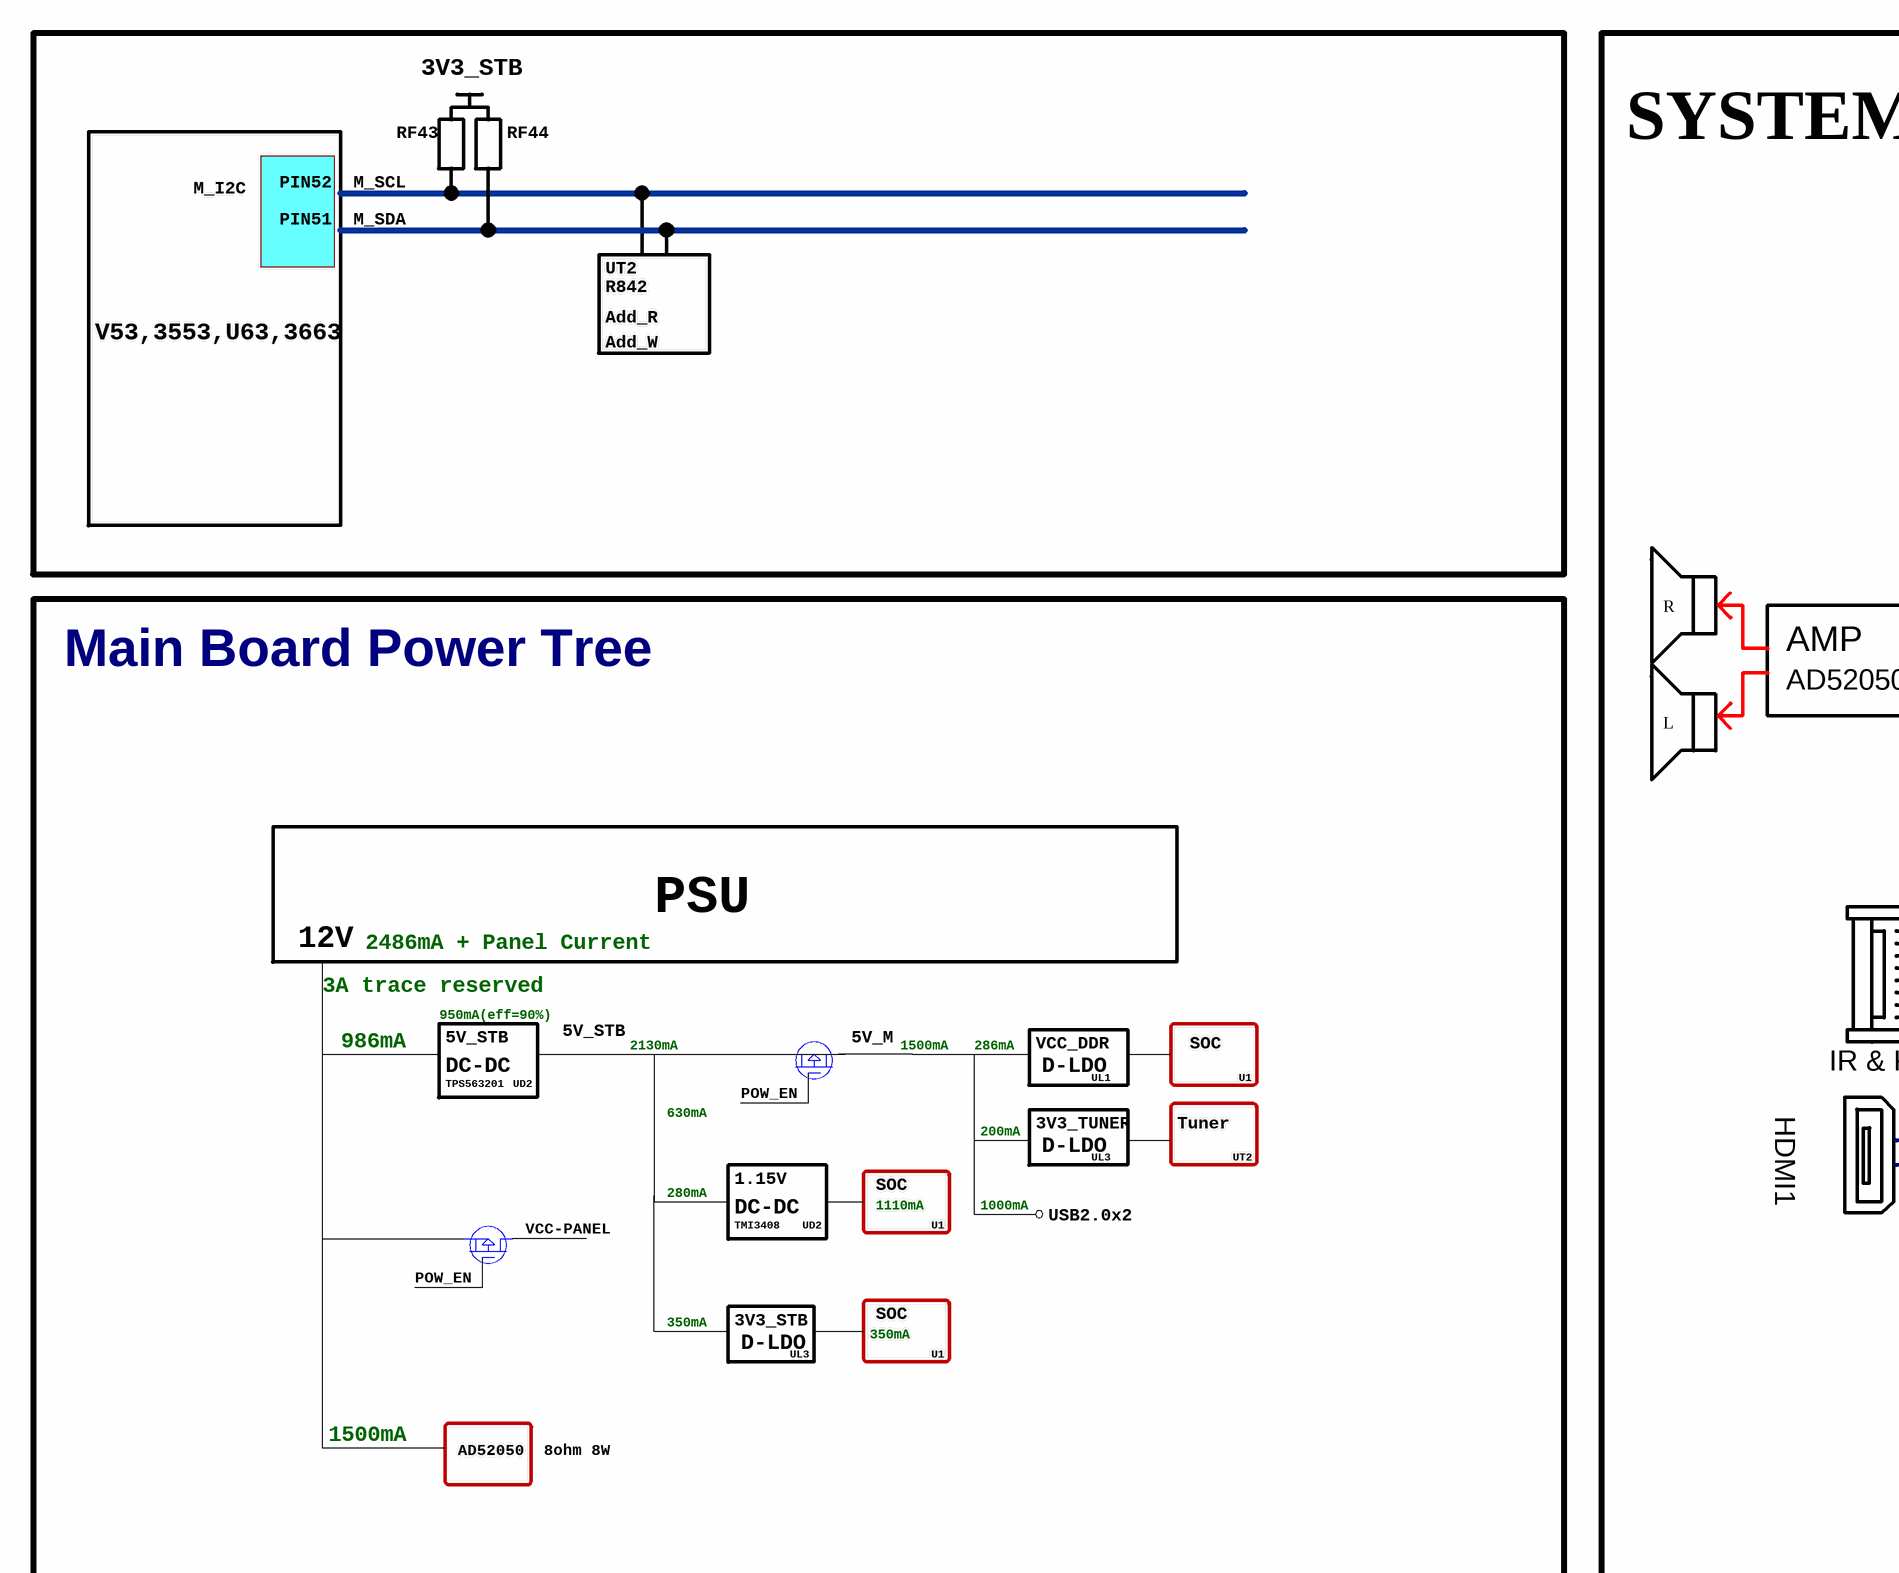
[diagram p0: MISC116569-14.SchDoc, left]
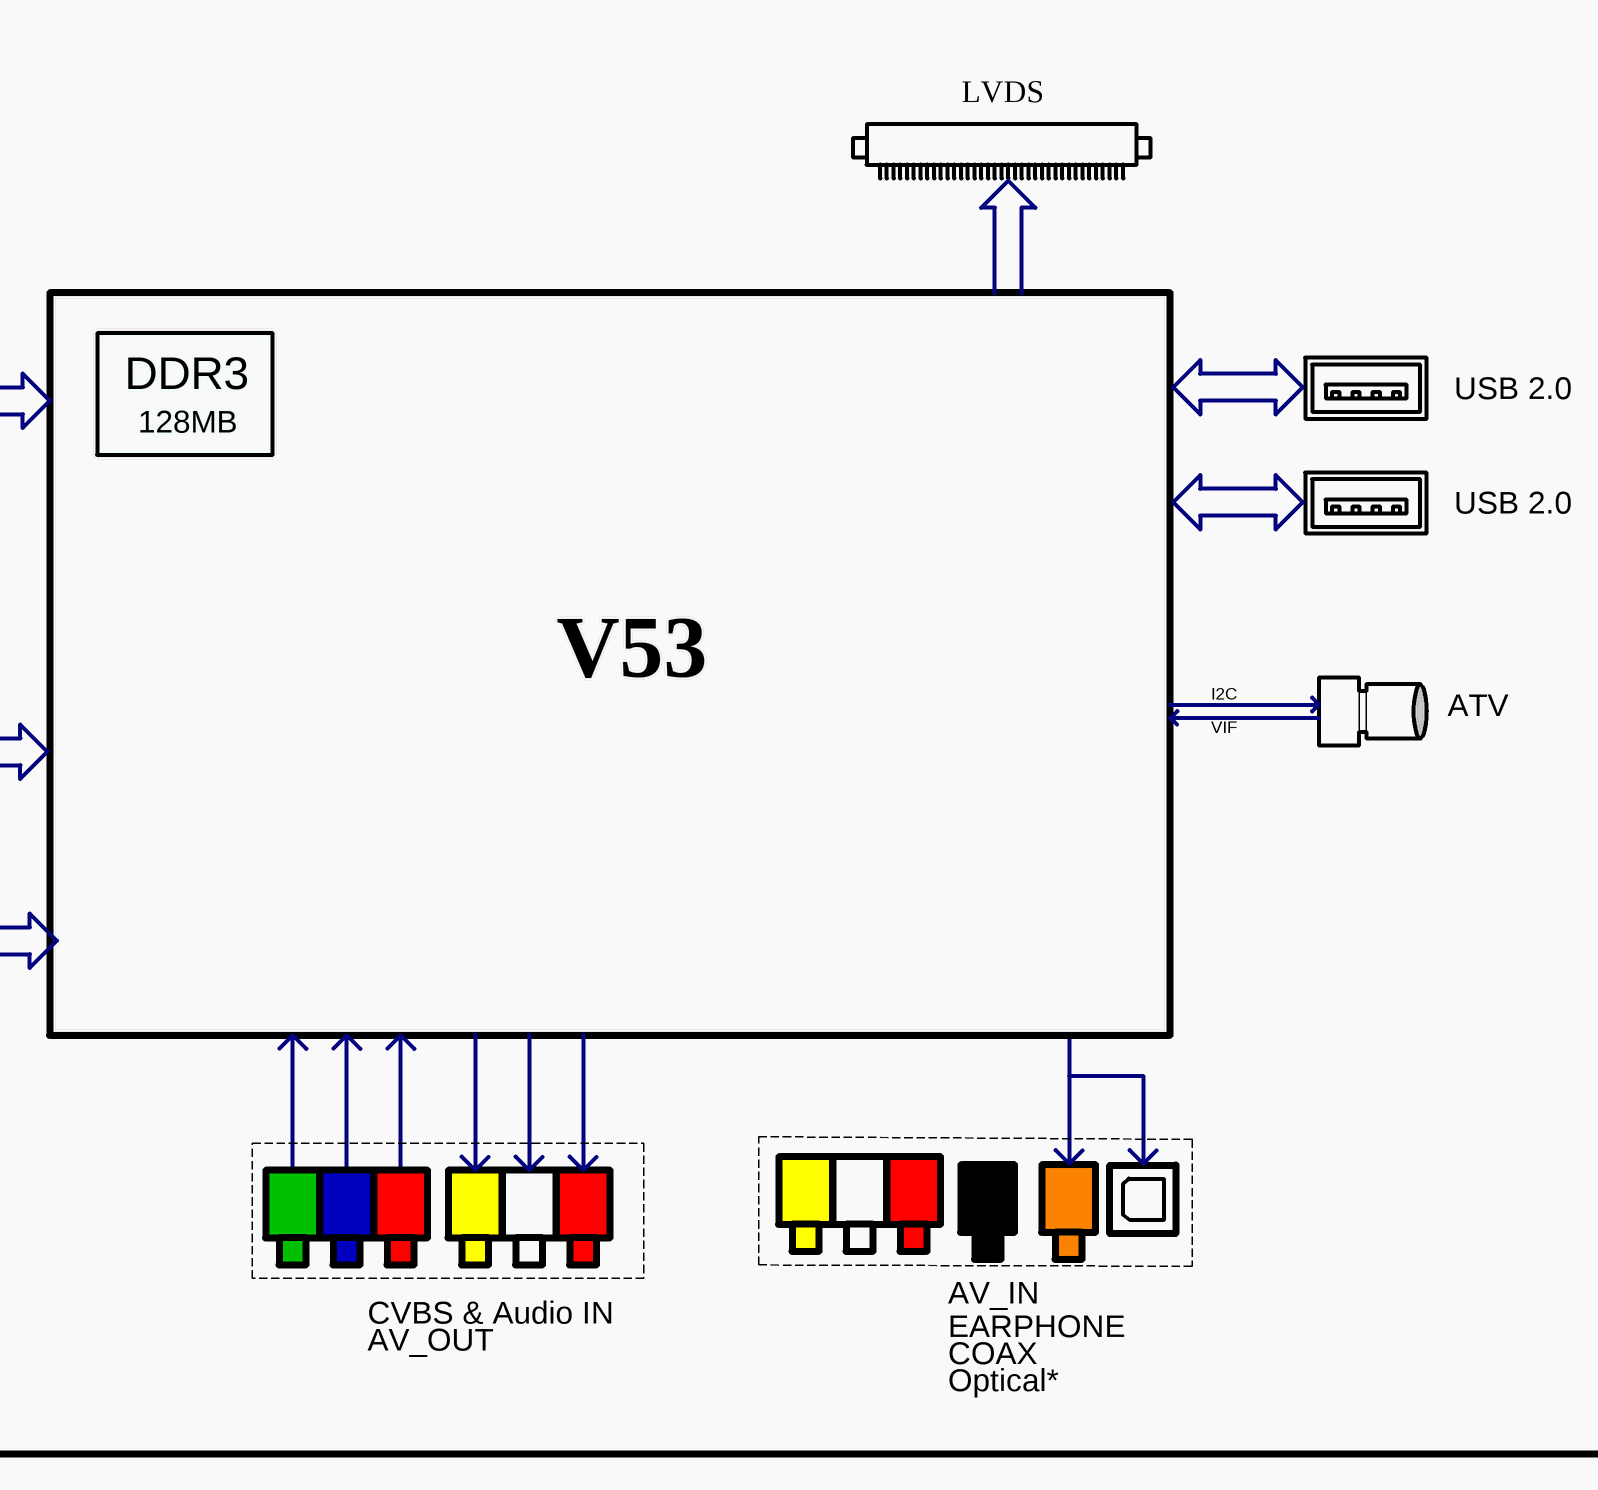
[diagram p1: MISC116569-14.SchDoc, right]
# Altium project MISC116569-15.PrjPCB (part 2 of 8)

## Sheet MISC116569-14.SchDoc
size 736 x 347 mm

### Notes on the sheet
- 3V3_STB
- RF43
- RF44
- SYSTEM FUNCTION BLOCK DIAGRAM
- M_I2C
- PIN52
- M_SCL
- PIN51
- M_SDA
- UT2
- V53,3553,U63,3663
- R842
- Add_R
- Add_W
- LVDS
- R
- Main Board Power Tree
- AMP
- AD52050
- DDR3
- 128MB
- USB 2.0
- L
- 12V
- 2486mA + Panel Current
- PSU
- V53
- I2C
- ATV
- 3A trace reserved
- VIF
- 986mA
- 950mA(eff=90%)
- DC-DC
- 5V_STB
- 2130mA
- 5V_M
- 1500mA
- 286mA
- VCC_DDR
- D-LDO
- UL1
- SOC
- U1
- IR & KEY
- TPS563201
- UD2
- 630mA
- POW_EN
- 200mA
- 3V3_TUNER
- Tuner
- HDMI1
- 280mA
- 1.15V
- UL3
- VCC-PANEL
- TMI3408
- 1110mA
- 1000mA
- USB2.0x2
- 350mA
- 8ohm 8W
- CVBS & Audio IN
- AV_IN
- AV_OUT
- COAX
- Optical*
- EARPHONE

## Sheet MISC116569-6.SchDoc
size 388 x 349 mm
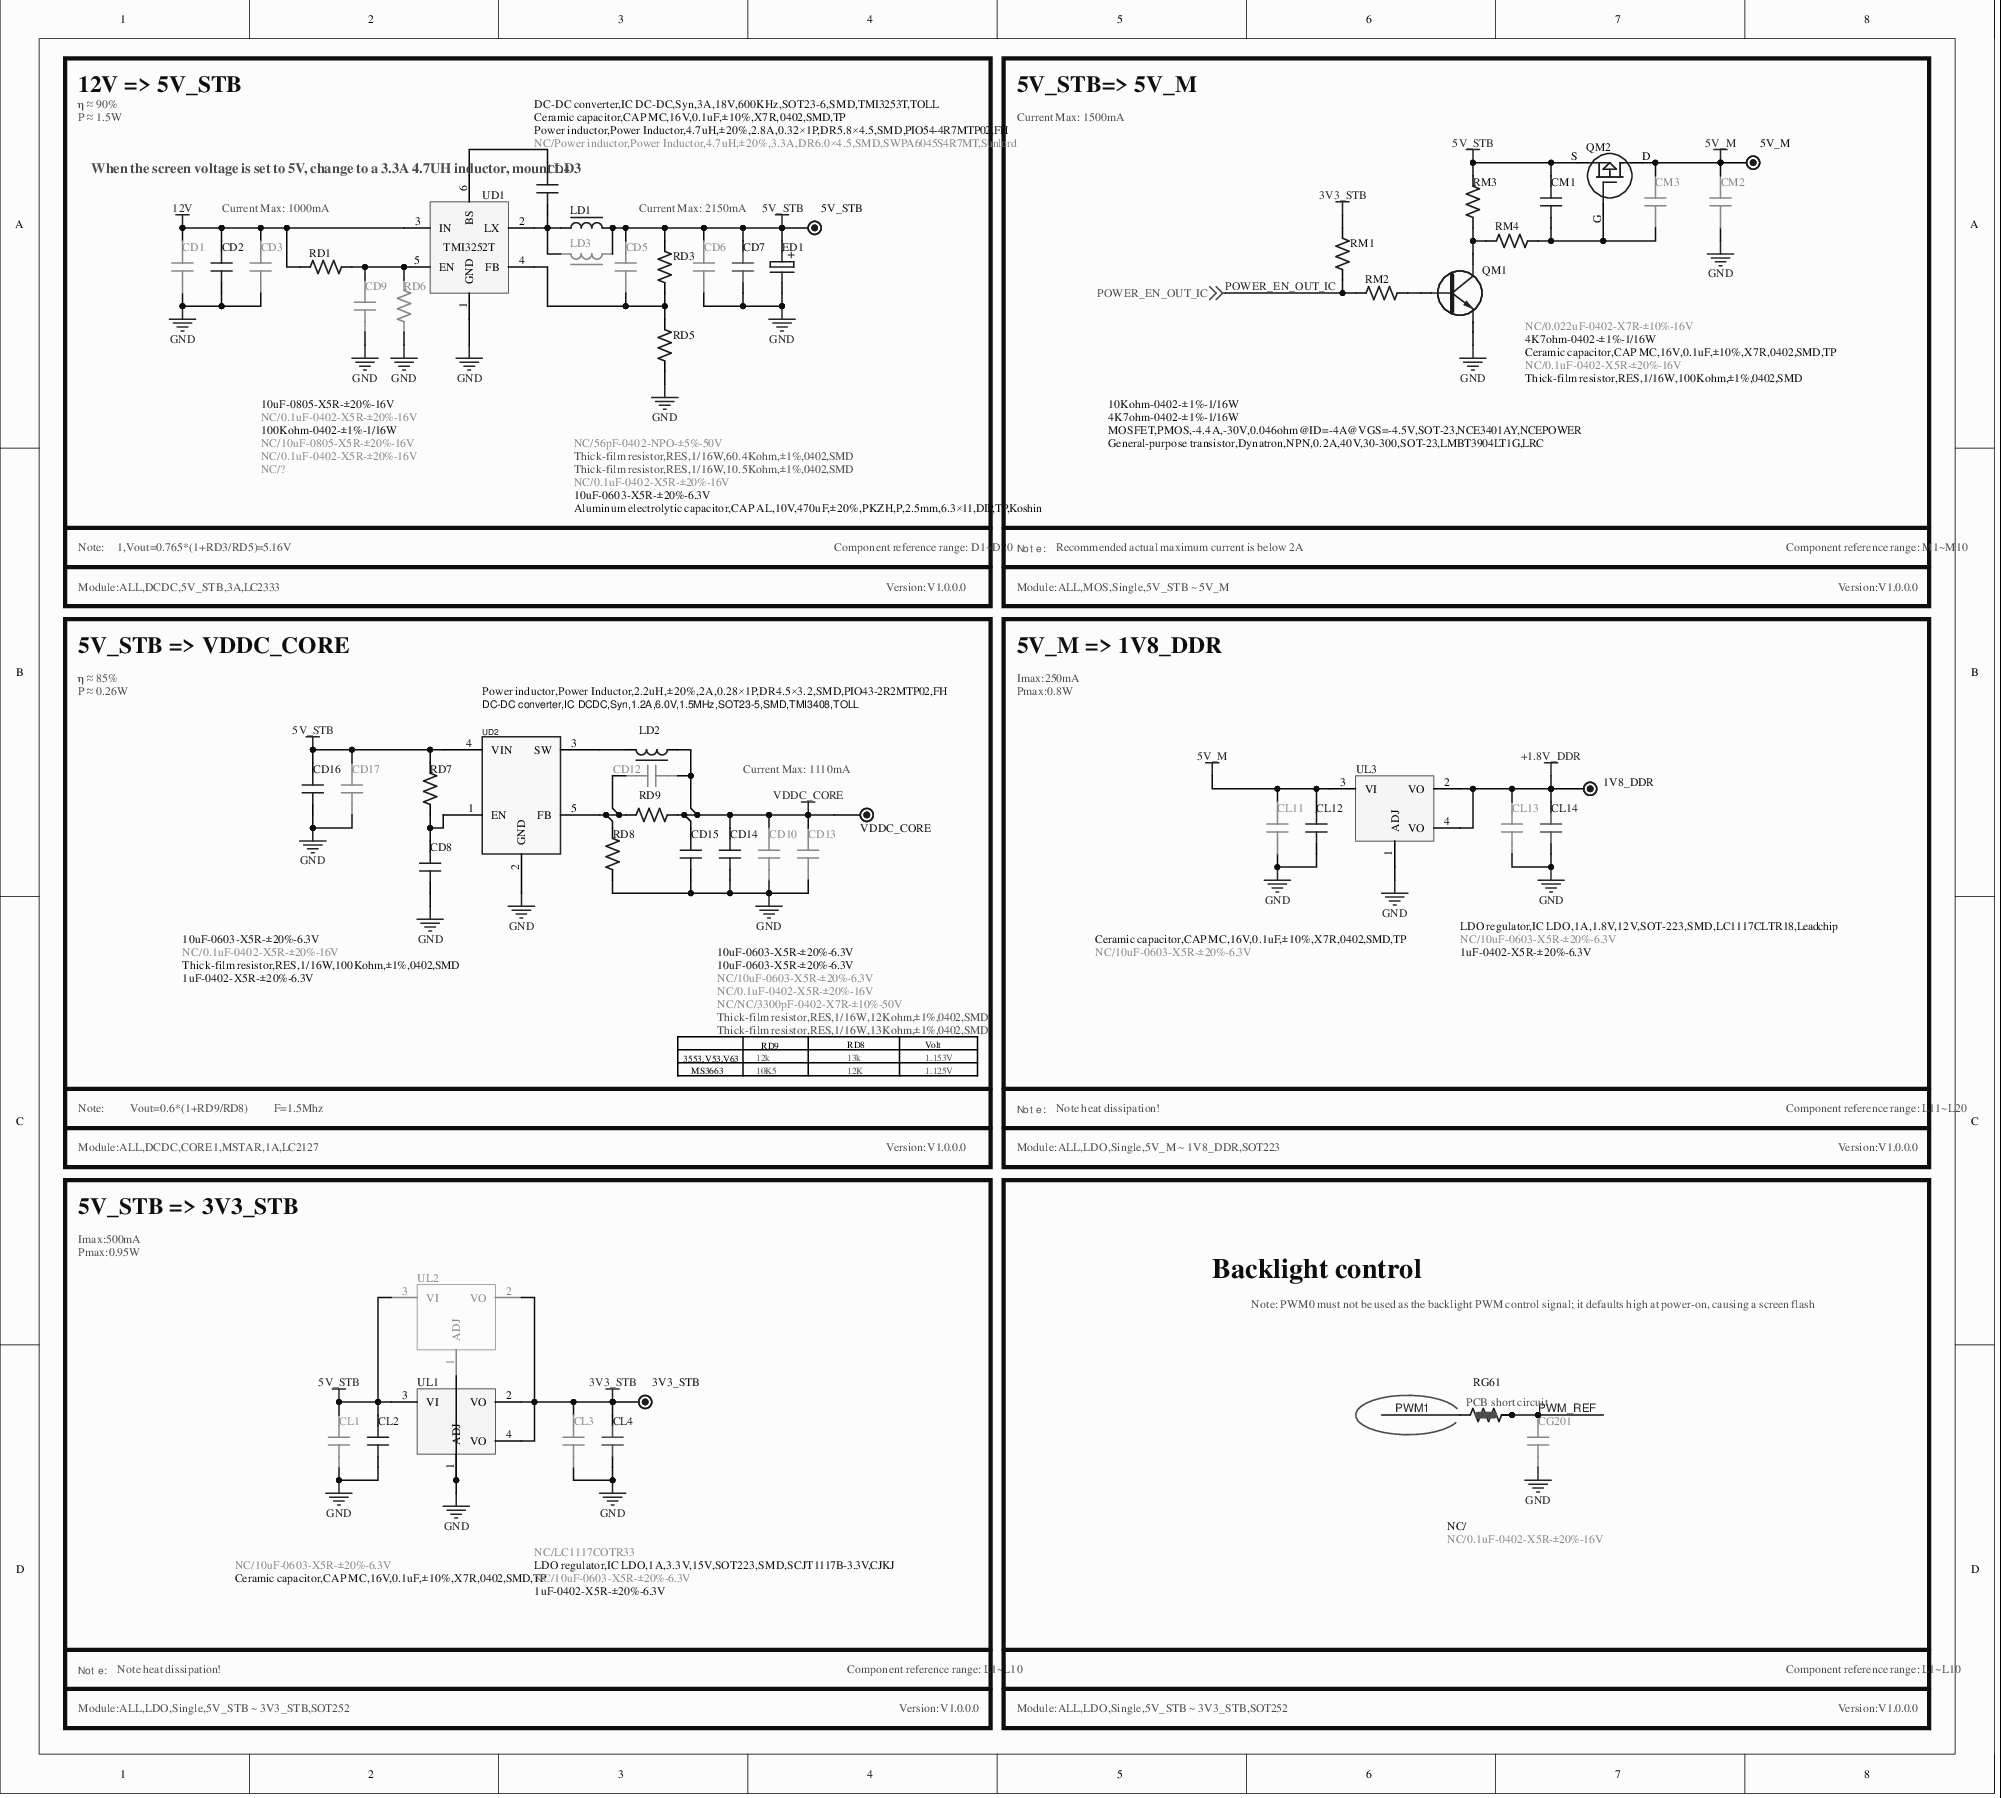
[diagram p2: MISC116569-6.SchDoc]

### Parts
1V8_DDR  TEST  [TP]  (value not drawn)
3V3_STB  TEST  [TP]  (value not drawn)
5V_M  TEST  [TP]  (value not drawn)
5V_STB  TEST  [TP]  (value not drawn)
CD1  NC/10uF-0805-X5R-±20%-16V  [C0805]
CD2  10uF-0805-X5R-±20%-16V  [C0805]
CD3  NC/0.1uF-0402-X5R-±20%-16V  [C0402]
CD4  Ceramic capacitor,CAP MC,16V,0.1uF,±10%,X7R,0402,SMD,TP  [C0402]
CD5  NC/56pF-0402-NPO-±5%-50V  [C0402]
CD6  NC/0.1uF-0402-X5R-±20%-16V  [C0402]
CD7  10uF-0603-X5R-±20%-6.3V  [C0603]
CD8  1uF-0402-X5R-±20%-6.3V  [C0402]
CD9  NC/0.1uF-0402-X5R-±20%-16V  [C0402]
CD10  NC/10uF-0603-X5R-±20%-6.3V  [C0603]
CD12  NC/NC/3300pF-0402-X7R-±10%-50V  [C0402]
CD13  NC/0.1uF-0402-X5R-±20%-16V  [C0402]
CD14  10uF-0603-X5R-±20%-6.3V  [C0603]
CD15  10uF-0603-X5R-±20%-6.3V  [C0603]
CD16  10uF-0603-X5R-±20%-6.3V  [C0603]
CD17  NC/0.1uF-0402-X5R-±20%-16V  [C0402]
CG201  NC/0.1uF-0402-X5R-±20%-16V  [C0402]
CL1  NC/10uF-0603-X5R-±20%-6.3V  [C0603]
CL2  Ceramic capacitor,CAP MC,16V,0.1uF,±10%,X7R,0402,SMD,TP  [C0402]
CL3  NC/10uF-0603-X5R-±20%-6.3V  [C0603]
CL4  1uF-0402-X5R-±20%-6.3V  [C0402]
CL11  NC/10uF-0603-X5R-±20%-6.3V  [C0603]
CL12  Ceramic capacitor,CAP MC,16V,0.1uF,±10%,X7R,0402,SMD,TP  [C0402]
CL13  NC/10uF-0603-X5R-±20%-6.3V  [C0603]
CL14  1uF-0402-X5R-±20%-6.3V  [C0402]
CM1  Ceramic capacitor,CAP MC,16V,0.1uF,±10%,X7R,0402,SMD,TP  [C0402]
CM2  NC/0.1uF-0402-X5R-±20%-16V  [C0402]
CM3  NC/0.022uF-0402-X7R-±10%-16V  [C0402]
ED1  Aluminum electrolytic capacitor,CAP AL,10V,470uF,±20%,PKZH,P,2.5mm,6.3×11,DIP,TP,Koshin  [EC(6.3*11)-V-2.5]
LD1  Power inductor,Power Inductor,4.7uH,±20%,2.8A,0.32×1P,DR5.8×4.5,SMD,PIO54-4R7MTP02,FH  [L(5.8*4.5)-S]
LD2  Power inductor,Power Inductor,2.2uH,±20%,2A,0.28×1P,DR4.5×3.2,SMD,PIO43-2R2MTP02,FH  [L(4.5*3.5)-S]
LD3  NC/Power inductor,Power Inductor,4.7uH,±20%,3.3A,DR6.0×4.5,SMD,SWPA6045S4R7MT,Sunlord  [L(6.0*4.5)-S]
QM1  General-purpose transistor,Dynatron,NPN,0.2A,40V,30-300,SOT-23,LMBT3904LT1G,LRC  [SOT-23]
QM2  MOSFET,PMOS,-4.4A,-30V,0.046ohm@ID=-4A@VGS=-4.5V,SOT-23,NCE3401AY,NCEPOWER  [SOT-23-1]
RD1  100Kohm-0402-±1%-1/16W  [R0402]
RD3  Thick-film resistor,RES,1/16W,60.4Kohm,±1%,0402,SMD  [R0402]
RD5  Thick-film resistor,RES,1/16W,10.5Kohm,±1%,0402,SMD  [R0402]
RD6  NC/?  [R0402]
RD7  Thick-film resistor,RES,1/16W,100Kohm,±1%,0402,SMD  [R0402]
RD8  Thick-film resistor,RES,1/16W,13Kohm,±1%,0402,SMD  [R0402]
RD9  Thick-film resistor,RES,1/16W,12Kohm,±1%,0402,SMD  [R0402]
RG61  NC/  [R0402SC]
RM1  10Kohm-0402-±1%-1/16W  [R0402]
RM2  4K7ohm-0402-±1%-1/16W  [R0402]
RM3  4K7ohm-0402-±1%-1/16W  [R0402]
RM4  Thick-film resistor,RES,1/16W,100Kohm,±1%,0402,SMD  [R0402]
UD1  DC-DC converter,IC DC-DC,Syn,3A,18V,600KHz,SOT23-6,SMD,TMI3253T,TOLL  [TSOT23-6]
UD2  DC-DC converter,IC DCDC,Syn,1.2A,6.0V,1.5MHz,SOT23-5,SMD,TMI3408,TOLL  [SOT-23-5]
UL1  LDO regulator,IC LDO,1A,3.3V,15V,SOT223,SMD,SCJT1117B-3.3V,CJKJ  [SOT-223]
UL2  NC/LC1117COTR33  [TO-252]
UL3  LDO regulator,IC LDO,1A,1.8V,12V,SOT-223,SMD,LC1117CLTR18,Leadchip  [SOT-223]
VDDC_CORE  TEST  [TP]  (value not drawn)

### Blocks framed on the sheet
12V => 5V_STB: 5V_STB CD1-CD7 CD9 ED1 LD1 LD3 RD1 RD3 RD5 RD6 UD1
5V_STB=> 5V_M: 5V_M CM1-CM3 QM1 QM2 RM1-RM4
5V_STB => VDDC_CORE: CD8 CD10 CD12-CD17 LD2 RD7-RD9 UD2 VDDC_CORE
5V_M => 1V8_DDR: 1V8_DDR CL11-CL14 UL3
5V_STB => 3V3_STB: 3V3_STB CL1-CL4 UL1 UL2
Backlight control: CG201 RG61

### Nets
3V3_STB: 3V3_STB.1 CL3.2 CL4.2 RM1.2 UL1.2(VO) UL1.4(VO) UL2.2(VO)
5V_M: 5V_M.1 CL11.2 CL12.2 CM2.2 CM3.1 QM2.D UL3.3(VI)
5V_STB: 5V_STB.1 CD5.2 CD6.2 CD7.2 CD16.2 CD17.2 CL1.2 CL2.2 CM1.2 ED1.1 LD1.2 LD3.1 QM2.S RD3.2 RD7.2 RM3.2 UD2.4(VIN) UL1.3(VI) UL2.3(VI)
12V: CD1.1 CD2.1 CD3.2 RD1.1 UD1.3(IN)
+1.8V_DDR: 1V8_DDR.1 CL13.2 CL14.2 UL3.2(VO) UL3.4(VO)
GND: CD1.2 CD2.2 CD3.1 CD6.1 CD7.1 CD8.1 CD9.1 CD10.1 CD13.1 CD14.1 CD15.1 CD16.1 CD17.1 CG201.2 CL1.1 CL2.1 CL3.1 CL4.1 CL11.1 CL12.1 CL13.1 CL14.1 CM2.1 ED1.2 QM1.E RD5.1 RD6.1 RD8.2 UD1.1(GND) UD2.2(GND) UL1.1(ADJ) UL2.1(ADJ) UL3.1(ADJ)
PWM_REF: CG201.1 RG61.2 RG61.3
VDDC_CORE: CD10.2 CD12.2 CD13.2 CD14.2 CD15.2 LD2.1 RD9.1 VDDC_CORE.1
POWER_EN_OUT_IC: RM1.1 RM2.1 ; off-sheet POWER_EN_OUT_IC
PWM1: RG61.1
NetCD4_1: CD4.1 LD1.1 LD3.2 UD1.2(LX)
NetCD4_2: CD4.2 UD1.6(BS)
NetCD5_1: CD5.1 RD3.1 RD5.2 UD1.4(FB)
NetCD8_2: CD8.2 RD7.1 UD2.1(EN)
NetCD9_2: CD9.2 RD1.2 RD6.2 UD1.5(EN)
NetCD12_1: CD12.1 RD8.1 RD9.2 UD2.5(FB)
NetCM1_1: CM1.1 CM3.2 QM2.G RM4.2
NetLD2_2: LD2.2 UD2.3(SW)
NetQM1_B: QM1.B RM2.2
NetQM1_C: QM1.C RM3.1 RM4.1

### Notes on the sheet
- η ≈ 90%
- P ≈ 1.5W
- Current Max: 1500mA
- (near CD4) When the screen voltage is set to 5V, change to a 3.3A 4.7UH inductor, mount LD3
- Current Max: 1000mA
- Current Max: 2150mA
- Note:
- 1,Vout=0.765*(1+RD3/RD5)=5.16V
- Component reference range: D1~D20
- Recommended actual maximum current is below 2A
- Component reference range: M1~M10
- Module:ALL,DCDC,5V_STB,3A,LC2333
- Version:V1.0.0.0
- Module:ALL,MOS,Single,5V_STB ~ 5V_M
- η ≈ 85%
- P ≈ 0.26W
- Pmax:0.8W
- Imax:250mA
- Current Max: 1110mA
- 3553,V53,V63
- MS3663
- 12k
- 10K5
- RD9
- RD8
- 13k
- 12K
- Volt
- 1.153V
- 1.125V
- Module:ALL,DCDC,CORE1,MSTAR,1A,LC2127
- Vout=0.6*(1+RD9/RD8)
- F=1.5Mhz
- Module:ALL,LDO,Single,5V_M ~ 1V8_DDR,SOT223
- Note heat dissipation!
- Component reference range: L11~L20
- Pmax:0.95W
- Imax:500mA
- Note: PWM0 must not be used as the backlight PWM control signal; it defaults high at power-on, causing a screen flash
- Component reference range: L1~L10
- Module:ALL,LDO,Single,5V_STB ~ 3V3_STB,SOT252

### Library data of the parts
CD1 CD2 = 004.003.0000386-D: Ceramic capacitor,CAP MC,16V,10uF,±20%,X5R,0805,SMD,TP-D
CD3 CD4 CD6 CD8 CD9 CL2 CL12 CM1 CM2 = 004.003.0000403-D: Ceramic capacitor,CAP MC,16V,0.1uF,±20%,X5R,0402,SMD,TP-D
CD5 = 004.003.0000570-D: Ceramic capacitor,CAP MC,50V,56pF,±5%,NPO,0402,SMD,TP-D
CD7 CL13 = 004.003.0000383-D: Ceramic capacitor,CAP MC,6.3V,10uF,±20%,X5R,0603,SMD,TP-D
CD10 CD14-CD16 CL1 CL3 CL11 = 10uF-0603-X5R-±20%-6.3V-D
CD12 = 3300pF-0402-X7R-±10%-50V-D
CD13 CD17 = 0.1uF-0402-X5R-±20%-16V-D
CG201 = 0.1uF-0402-Y5V-+80%-20%-16V-D
CL4 CL14 = 004.003.0000382-D: Ceramic capacitor,CAP MC,6.3V,1uF,±20%,X5R,0402,SMD,TP-D
CM3 = 0.022uF-0402-X7R-±10%-16V-D
ED1 = 470uF-10V-±20%-6.3×11-105℃-黑底白字-编带-F=2.5-XF-DHAI: Electrolytic
LD1 = 004.004.0000017-D: Power inductor,Power Inductor,4.7uH,±20%,2.8A,0.35×1P,DR5.8×4.5,SMD,SCD54TL-4R7M,Soldier-D
LD2 = SLN43T-6R8M-D
LD3 = 004.004.0000016-D: Power inductor,Power Inductor,4.7uH,±20%,3.3A,DR6.0×4.5,SMD,SWPA6045S4R7MT,Sunlord-D
QM1 = 004.006.0000007-D: General-purpose transistor,Dynatron,NPN,0.2A,40V,60-300,SOT-23,KMBT3904,KEXIN-D
QM2 = 004.007.0000286-D: MOSFET,PMOS,-4.7A,-20V,70mohm@ID=-4.7A@VGS=-4.5V,SOT23-LC,LPB3443LT1G,LRC-D
RD1 RD7 RM4 = 004.002.0000579-D: Thick-film resistor,RES,1/16W,100Kohm,±5%,0402,SMD-D
RD3 = 004.002.0000104-D: Thick-film resistor,RES,1/16W,33Kohm,±1%,0402,SMD-D
RD5 = 004.002.0000717-D: Thick-film resistor,RES,1/16W,6.04Kohm,±1%,0402,SMD-D
RD6 = 004.002.0000806-D: Thick-film resistor,RES,1/16W,60.4Kohm,±1%,0402,SMD-D
RD8 = 004.002.0000593-D: Thick-film resistor,RES,1/16W,13Kohm,±1%,0402,SMD-D
RD9 = 004.002.0000588-D: Thick-film resistor,RES,1/16W,12Kohm,±1%,0402,SMD-D
RG61 = 0ohm-0402-PCB-D
RM1 RM2 = 004.002.0000577-D: Thick-film resistor,RES,1/16W,10Kohm,±5%,0402,SMD-D
RM3 = 004.002.0000689-D: Thick-film resistor,RES,1/16W,4.7Kohm,±5%,0402,SMD-D
UD1 = 004.010.0001184-D: DC-DC converter,IC DC-DC,Syn,2A,18V,600KHz,SOT23-6,SMD,TMI3252T,TOLL-D
UD2 = DC-DC芯片,IC DCDC,Syn,1.2A,7.0V,1.5MHz,SOT23-5,SMD,LC2127CB5TR,Leadchip-D
UL1 UL3 = 004.010.0000061-D: LDO regulator,IC LDO,1A,1.8V,12V,SOT-223,SMD,LC1117CLTR18,Leadchip-D
UL2 = 004.010.0000064-D: LDO regulator,IC LDO,1A,3.3V,12V,TO-252,SMD,LC1117COTR33,Leadchip-D